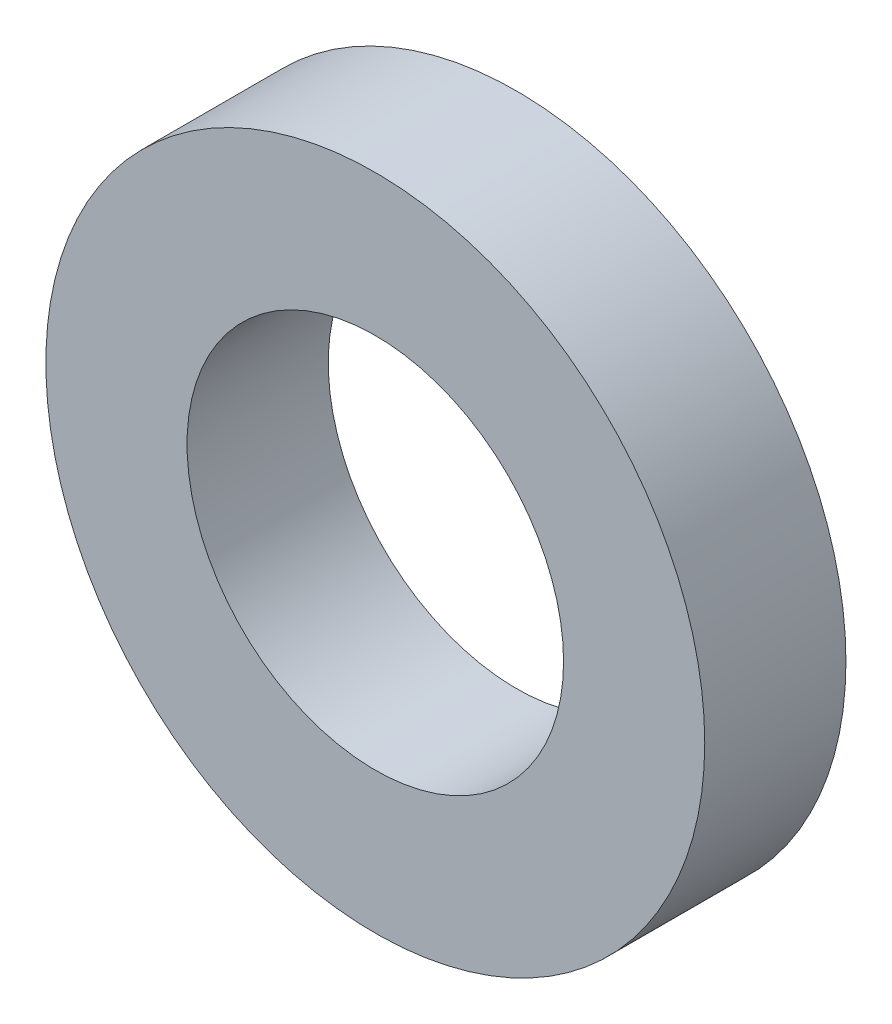
SolidWorks part; units mm, degrees
material "Q235B"
ref_plane "Front Plane" through (0, 0, 0) normal (0, 0, 1) x (1, 0, 0)
ref_plane "Top Plane" through (0, 0, 0) normal (0, 1, 0) x (1, 0, 0)
ref_plane "Right Plane" through (0, 0, 0) normal (1, 0, 0) x (0, 0, -1)
sketch "Sketch1" plane through (0, 0, 0) normal (0, 0, 1) x (1, 0, 0)
  circle A0 centre (0, 0) radius 35
  circle A1 centre (0, 0) radius 20
  dimension "D1" = 70
  dimension "D2" = 40
extrude "Boss-Extrude1" add sketch "Sketch1" along normal blind 15
